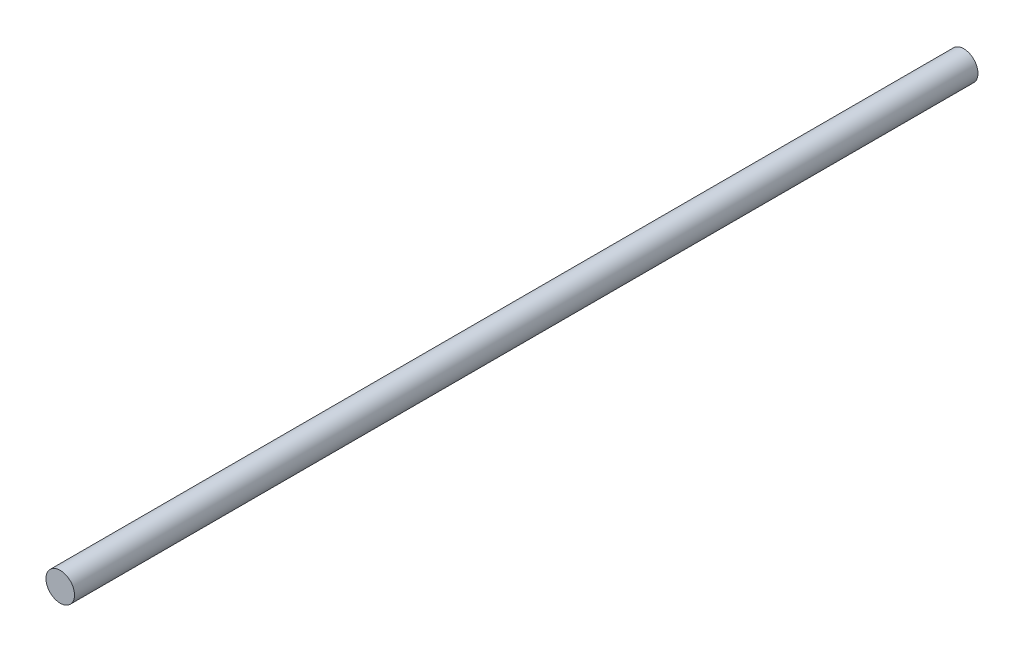
from build123d import *

# Parameters (mm, degrees)
SKETCH_1_R      = 6
EXTRUDE_1_DEPTH = 190


with BuildPart() as part:
    # 草图1 → 凸台-拉伸1 (new, symmetric)
    with BuildSketch(Plane.XY):
        Circle(SKETCH_1_R)
    extrude(amount=EXTRUDE_1_DEPTH, both=True)


solid = part.part
